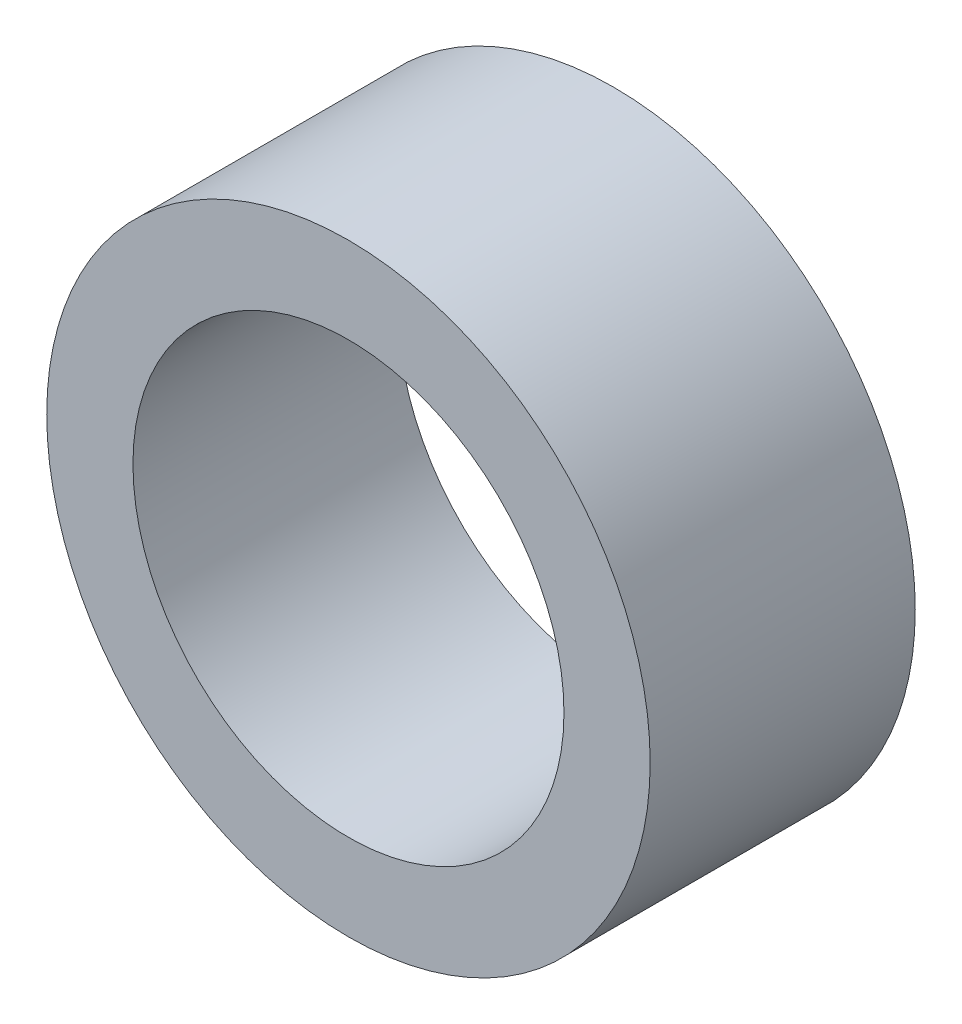
SolidWorks part; units mm, degrees
ref_plane "前视基准面" through (0, 0, 0) normal (0, 0, 1) x (1, 0, 0)
ref_plane "上视基准面" through (0, 0, 0) normal (0, 1, 0) x (1, 0, 0)
ref_plane "右视基准面" through (0, 0, 0) normal (1, 0, 0) x (0, 0, -1)
sketch "草图1" plane through (0, 0, 0) normal (0, 0, 1) x (1, 0, 0)
  circle A0 centre (0, 0) radius 5
  circle A1 centre (0, 0) radius 7
  dimension "D1" = 10
  dimension "D2" = 14
extrude "凸台-拉伸1" add sketch "草图1" along normal blind 6.15
